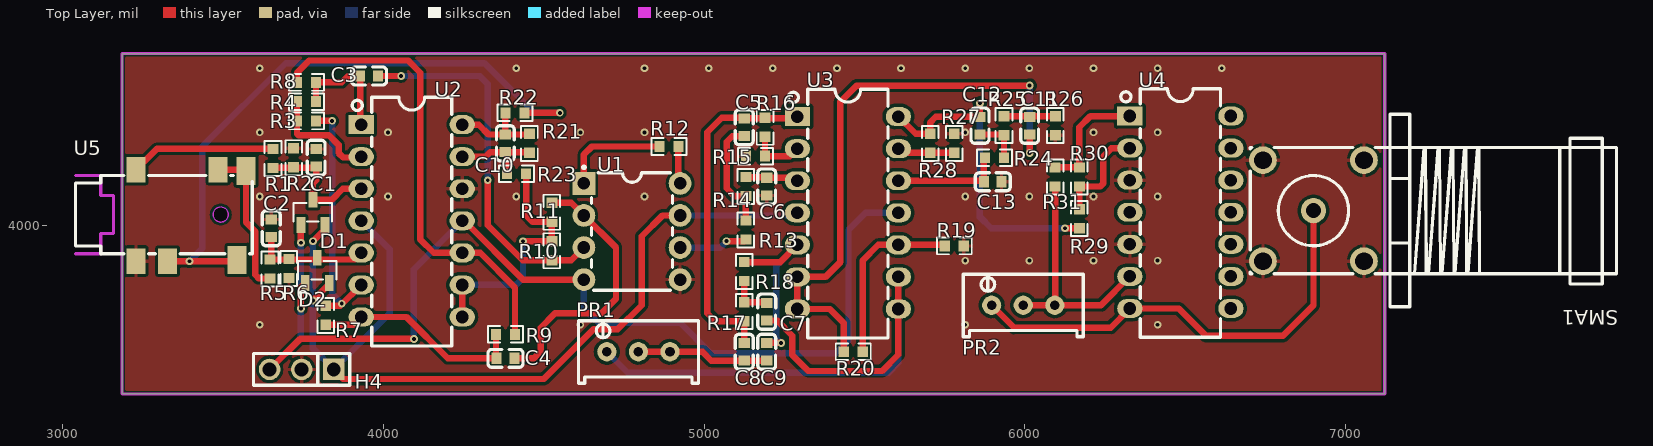
[diagram p0: Top Layer view]
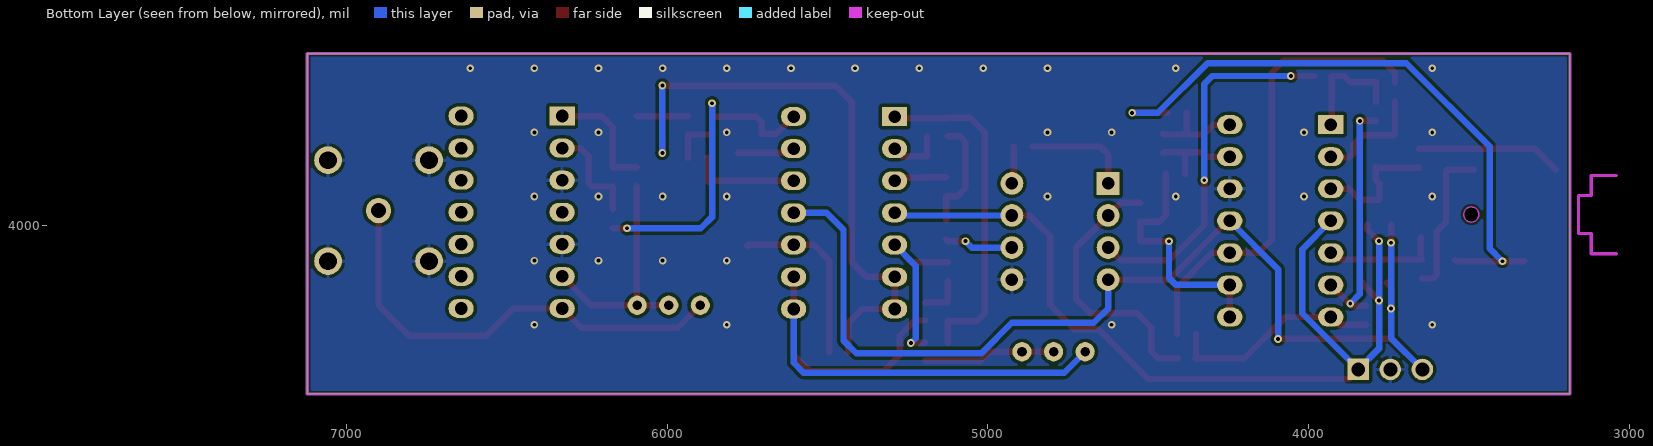
[diagram p1: Bottom Layer view, seen from below]
# Altium PCB MISC51578.pcbdoc
Units mil, origin at the board's own origin, x right, y up, seen from the top; angles counter-clockwise.
Board outline 3937.01 x 1061.35 mil, 2 copper layers (Top Layer, Bottom Layer), stack 62.206 mil thick; 55 components, 40 nets, 164 pads, 53 vias.

## Layer stack, top to bottom
Top Solder Mask Layer: solder mask 0.394, Dk 3.3
Top Layer: signal copper 1.379
Dielectric1: surface 59.449, FR4, Dk 4.5
Bottom Layer: signal copper 1.378
Bottom Solder Mask Layer: solder mask 0.394, Dk 3.3

## Board outline
3185,4535 3185,3473.65 7122.01,3473.65 7122.01,4535

## Design rules (kind name [scope] priority, off if disabled: settings)
BoardOutlineClearance copperThickness2oz_1 [All] p2 off: genericclearance=7.99 ignorepadtopadclearanceinfootprint=FALSE except(0: Arc-SplitContinuation Track-SplitContinuation SMDPad-SplitContinuation THPad-SplitContinuation Via-SplitContinuation Fill-SplitContinuation Region-SplitContinuation Poly-SplitContinuation Text-SplitContinuation Hole-SplitContinuation; 5.98: Arc-CutoutEdge SMDPad-CutoutEdge THPad-CutoutEdge Via-CutoutEdge Fill-CutoutEdge Region-CutoutEdge Text-CutoutEdge; 6.93: Hole-OutlineEdge Hole-CutoutEdge; 10: Poly-OutlineEdge Poly-CutoutEdge; 11.81: Arc-OutlineEdge Track-OutlineEdge SMDPad-OutlineEdge THPad-OutlineEdge Via-OutlineEdge Fill-OutlineEdge Region-OutlineEdge Text-OutlineEdge Track-CutoutEdge)
BoardOutlineClearance copperThickness1oz_1 [All] p4: genericclearance=4.02 ignorepadtopadclearanceinfootprint=FALSE except(0: Arc-SplitContinuation Track-SplitContinuation SMDPad-SplitContinuation THPad-SplitContinuation Via-SplitContinuation Fill-SplitContinuation Region-SplitContinuation Poly-SplitContinuation Text-SplitContinuation Hole-SplitContinuation; 6: SMDPad-CutoutEdge THPad-CutoutEdge Via-CutoutEdge Fill-CutoutEdge Region-CutoutEdge Text-CutoutEdge; 6.93: Hole-OutlineEdge Hole-CutoutEdge; 10: Poly-OutlineEdge Poly-CutoutEdge; 11.8: Arc-OutlineEdge Track-OutlineEdge SMDPad-OutlineEdge THPad-OutlineEdge Via-OutlineEdge Fill-OutlineEdge Region-OutlineEdge Text-OutlineEdge; 11.81: Arc-CutoutEdge Track-CutoutEdge)
Clearance copperThickness2oz [All] p1 off: gap=7.99 ignorepadtopadclearanceinfootprint=FALSE except(5.98: SMDPad-Track SMDPad-SMDPad THPad-Track SMDPad-THPad THPad-THPad Track-Via SMDPad-Via THPad-Via Via-Via Fill-Track Region-Track Fill-SMDPad Region-SMDPad Fill-THPad Region-THPad Fill-Via Region-Via Fill-Fill Fill-Region Region-Region Arc-Track Arc-SMDPad Arc-THPad Arc-Via Fill-Arc Region-Arc Arc-Arc Text-Track SMDPad-Text Text-THPad Text-Via Fill-Text Region-Text Arc-Text Text-Text; 6.93: Hole-Track Hole-SMDPad Hole-THPad Hole-Via Fill-Hole Region-Hole Hole-Arc Hole-Text; 10: Poly-Track Poly-SMDPad Poly-THPad Poly-Via Poly-Fill Poly-Region Poly-Poly Poly-Arc Poly-Text Poly-Hole)
Clearance copperThickness1oz [All] p3: gap=4.02 ignorepadtopadclearanceinfootprint=FALSE except(5.98: SMDPad-Track SMDPad-SMDPad THPad-Track SMDPad-THPad THPad-THPad Track-Via SMDPad-Via THPad-Via Via-Via Fill-Track Region-Track Fill-SMDPad Region-SMDPad Fill-THPad Region-THPad Fill-Via Region-Via Fill-Fill Fill-Region Region-Region; 6: Arc-Track Arc-SMDPad Arc-THPad Arc-Via Fill-Arc Region-Arc Arc-Arc Text-Track SMDPad-Text Text-THPad Text-Via Fill-Text Region-Text Arc-Text Text-Text; 6.93: Hole-Track Hole-SMDPad Hole-THPad Hole-Via Fill-Hole Region-Hole Hole-Arc Hole-Text; 10: Poly-Track Poly-SMDPad Poly-THPad Poly-Via Poly-Fill Poly-Region Poly-Poly Poly-Arc Poly-Text Poly-Hole)
DiffPairsRouting differentialPair [All] p1: maxlimit=6 minlimit=6 mostfreqgap=6 toplayer_minwidth=5 toplayer_prefwidth=10 toplayer_maxwidth=100 toplayer_mingap=6 toplayer_prefgap=6 toplayer_maxgap=6 bottomlayer_minwidth=5 bottomlayer_prefwidth=10 bottomlayer_maxwidth=100 bottomlayer_mingap=6 bottomlayer_prefgap=6 bottomlayer_maxgap=6 maxuncoupledlength=10
HoleToHoleClearance otherClearance [All] p1: gap=11.81 allowstackedmicrovias=TRUE
Length netLength [All] p1: minlimit=0 maxlimit=0
MatchedLengths netLengthTolerance [All] p1: tolerance=1000
PasteMaskExpansion pasteMaskExpansion [All] p1: expansion=0
PlaneConnect innerPlane [All] p1: planeconnectstyle=Relief reliefexpansion=20 reliefentries=4 reliefconductorwidth=10 reliefairgap=10
PolygonConnect copperRegion [(InNet('GND'))] p1: connectstyle=Relief reliefconductorwidth=10 reliefentries=4 polygonreliefangle="90 Angle" airgapwidth=10 via.connectstyle=Relief via.reliefconductorwidth=10 via.reliefentries=4 via.polygonreliefangle="90 Angle" via.airgapwidth=10
RoutingVias viaSize [All] p1: holewidth=12.01 width=24.02 viastyle="Through Hole" minholewidth=11.81 minwidth=19.68 maxholewidth=248.03 maxwidth=393.7
SolderMaskExpansion solderMaskExpansion [IsVia] p1: expansion=-1000 istentingtop=TRUE
SolderMaskExpansion solderMaskExpansion [All] p2: expansion=2 istentingtop=FALSE
Width copperThickness2oz_2 [All] p1 off: maxlimit=100 minlimit=8 preferedwidth=10
Width copperThickness1oz_2 [All] p2: maxlimit=100 minlimit=5 preferedwidth=10

## Components (designator, comment, footprint, x,y, rotation, side; value= is the part's Value field where it differs from the comment)
C1 "1nF" C0603 3790,4210 r270 top
C2 "1nF" C0603 3650,3990 r270 top
C3 "330nF" C0603 3955,4465 r0 top
C4 "330nF" C0603 4380.52,3584.47 r0 top
C5 "470nF" C0603 5125,4305 r90 top
C6 "470nF" C0603 5195,4120 r90 top
C7 "220nF" C0603 5195,3730 r90 top
C8 "100nF" C0603 5125,3605 r90 top
C9 "100nF" C0603 5195,3605 r270 top
C10 "22nF" C0603 4380,4255 r270 top
C11 "100nF" C0603 6015,4310 r270 top
C12 "470nF" C0603 5860,4310 r270 top
C13 "470nF" C0603 5900,4135 r180 top
D1 "BAV99" SOT-23-3_L2.9-W1.3-P1.90-LS2.4-BR 3780,4040 r270 top
D2 "BAV99" SOT-23-3_L2.9-W1.3-P1.90-LS2.4-BR 3793.75,3858.98 r270 top
H4 "" HDR-TH_3P-P2.54-V-M 3745,3550 r180 top
PR1 "10kΩ" R_3296 4795,3610 r0 top
PR2 "20kΩ" R_3296 5995,3755 r0 top
R1 "51K" R0603 3655.56,4208.01 r270 top
R2 "10M" R0603 3720,4210 r90 top
R3 "20K" R0603 3760,4325 r180 top
R4 "10K" R0603 3760,4385 r180 top
R5 "51K" R0603 3646.24,3863.01 r90 top
R6 "10M" R0603 3705,3865 r270 top
R7 "10K" R0603 3820.04,3718.69 r90 top
R8 "20K" R0603 3760,4445 r0 top
R9 "20K" R0603 4380.52,3659.47 r0 top
R10 "10MΩ" R0603 4525,3920 r270 top
R11 "10MΩ" R0603 4525,4040 r270 top
R12 "5K" R0603 4890,4245 r0 top
R13 "15K" R0603 5130,3985 r90 top
R14 "15K" R0603 5130,4120 r90 top
R15 "10K" R0603 5160,4215 r0 top
R16 "10K" R0603 5190,4305 r270 top
R17 "30K" R0603 5125,3730 r90 top
R18 "30K" R0603 5125,3855 r90 top
R19 "10K" R0603 5780,3935 r180 top
R20 "5K" R0603 5465,3605 r180 top
R21 "10M" R0603 4455,4255 r270 top
R22 "1M" R0603 4410,4350 r180 top
R23 "10K" R0603 4415,4160 r0 top
R24 "15K" R0603 5905,4210 r0 top
R25 "15K" R0603 5935,4310 r90 top
R26 "1M" R0603 6095,4310 r90 top
R27 "10K" R0603 5780,4255 r270 top
R28 "10K" R0603 5705,4255 r90 top
R29 "2K" R0603 6170,4020 r270 top
R30 "20K" R0603 6170,4150 r270 top
R31 "2K" R0603 6094.66,4150.34 r90 top
SMA1 "BNC-9.6" SMA-TH_5P_BNC-9.6 6900,4045 r180 top
U1 "AD620ANZ" DIP-8_L9.3-W6.4-P2.54-LS7.6-BL 4775,3980 r270 top
U2 "LM324NG" PDIP-14_L19.7-W6.6-P2.54-LS8.3-BL 4088.16,4013.35 r270 top
U3 "LM324NG" PDIP-14_L19.7-W6.6-P2.54-LS8.3-BL 5448.22,4038.35 r270 top
U4 "LM324NG" PDIP-14_L19.7-W6.6-P2.54-LS8.3-BL 6485,4040 r270 top
U5 "PJ-342 earphone jack" AUDIO-SMD_PJ-342_C9900012319 3400,4030 r0 top

## Footprints (in the part's own frame and the unit in brackets; to place one, negate y for a bottom-side part, rotate by r counter-clockwise, add the part's x,y. Pads: shape width x height; smd on the part's side, far side on the other; paste and mask are expansions set on the pad)
AUDIO-SMD_PJ-342_C9900012319 [mm]
  rect 1.5x2 smd paste+0 mask+0.05: 2(-4.35,-3.625) 3(-4.35,3.625) 6(2.15,3.625) 7(-1.85,-3.625)
  rect 1.5x2.2 smd paste+0 mask+0.05: 4(4.35,3.525) 5(3.65,-3.525)
  Board Outline Layer circle w0.003: c2.35,0.075 r0.6
  Board Outline Layer lines w0.254: -9.15,-3.025 -7.15,-3.025 -7.15,-1.425 -6.15,-1.425 -6.151,1.576 -7.149,1.576 -7.149,3.174 -9.15,3.174
  Board Outline Layer region: 2.95,0.075 2.891,-0.185 2.724,-0.394 2.484,-0.51 2.216,-0.51 1.976,-0.394 1.809,-0.185 1.75,0.075 1.75,0.075 1.809,0.335 1.976,0.544 2.216,0.66 2.484,0.66 2.724,0.544 2.891,0.335 2.95,0.075
  Board Outline Layer region: 2.95,0.075 2.941,-0.029 2.914,-0.13 2.87,-0.225 2.81,-0.311 2.736,-0.385 2.65,-0.445 2.555,-0.489 2.454,-0.516 2.35,-0.525 2.246,-0.516 2.145,-0.489 2.05,-0.445 1.964,-0.385 1.89,-0.311 1.83,-0.225 1.786,-0.13 1.759,-0.029 1.75,0.075 1.759,0.179 1.786,0.28 1.83,0.375 1.89,0.461 1.964,0.535 2.05,0.595 2.145,0.639 2.246,0.666 2.35,0.675 2.454,0.666 2.555,0.639 2.65,0.595 2.736,0.535 2.81,0.461 2.87,0.375 2.914,0.28 2.941,0.179
  Multi-Layer board cut-out: 2.95,0.075 2.891,-0.185 2.724,-0.394 2.484,-0.51 2.216,-0.51 1.976,-0.394 1.809,-0.185 1.75,0.075 1.75,0.075 1.809,0.335 1.976,0.544 2.216,0.66 2.484,0.66 2.724,0.544 2.891,0.335 2.95,0.075
  silkscreen extent -9.15,-3.03 4.85,3.17
C0603 [mm]
  rect 0.8x0.9 smd: 1(-0.7,0) 2(0.7,0)
  silkscreen extent -1.39,-0.71 1.39,0.71
DIP-8_L9.3-W6.4-P2.54-LS7.6-BL [mm]
  rect 1.8x1.8 hole 1: 1(-3.81,-3.81)
  round 1.8 hole 1: 2(-1.27,-3.81) 3(1.27,-3.81) 4(3.81,-3.81) 5(3.81,3.81) 6(1.27,3.81) 7(-1.27,3.81) 8(-3.81,3.81)
  silkscreen extent -5.18,-3.91 4.65,3.2
HDR-TH_3P-P2.54-V-M [mm]
  rect 1.7x1.7 hole 1.1: 1(-2.54,0)
  round 1.7 hole 1.1: 2(0,0) 3(2.54,0)
  silkscreen extent -3.81,-1.25 3.81,1.25
PDIP-14_L19.7-W6.6-P2.54-LS8.3-BL [mm]
  rect 1.5x2 hole 1: 1(-7.62,-4)
  oval 1.5x2 hole 1: 2(-5.08,-4) 3(-2.54,-4) 4(0,-4) 5(2.54,-4) 6(5.08,-4) 7(7.62,-4) 8(7.62,4) 9(5.08,4) 10(2.54,4) 11(0,4) 12(-2.54,4) 13(-5.08,4) 14(-7.62,4)
  silkscreen extent -9.78,-4.72 9.91,3.18
R0603 [mil]
  rect 31.75x34.02 smd paste-3937.01 mask+2: 1(-29.66,0) 2(29.66,0)
  silkscreen extent -55,-26 55,26
R_3296 [mil]
  round 60 hole 30 paste+0 mask+2: 1(-98.4,-5) 2(0,-5) 3(98.4,-5)
  silkscreen extent -187,-103 187,92
SMA-TH_5P_BNC-9.6 [mm]
  round 2.2 hole 1.4 paste+0 mask+0.05: 1(-4,4) 2(4,4) 3(4,-4) 4(-4,-4)
  round 2 hole 1.2 paste+0 mask+0.05: 5(0,0)
  silkscreen extent -24,-7.63 5,7.62
SOT-23-3_L2.9-W1.3-P1.90-LS2.4-BR [mm]
  rect 1.25x0.7 smd: 1(1,-0.95) 2(1,0.95) 3(-1,0)
  silkscreen extent -0.73,-1.53 0.73,1.53

## Via types
v1: diameter 24.02, hole 12, Top Layer to Bottom Layer, 53 vias

## Nets (pads, with @x,y where several pads share a name; then routed paths per layer and width w, separated by ;. In a path a pad name is that pad's centre, name@x,y a point inside that pad or via, vN(x,y) a via of type N, cw(c..) or ccw(c..) an arc to the next point about the centre after c; other vN are vias at no path point)
12V: D1.2 D2.2 H4.1 U1.7 U2.4 U3.4 | length 2940.5
  Top Layer w20: v1(3780,3765) 3831.15,3816.15 D2.2 ; v1(3780,3950) 3817.4,3987.4 D1.2 ; H4.1 3875,3520 4500,3520 4655,3675 4730,3675 4805,3750 4805,3965 4870,4030 U1.7
  Bottom Layer w20: v1(3780,3950) v1(3780,3765) 3780,3615 H4.1 4020,3725 4020,3924.04 U2.4 ; U1.7 5282.38,4030 U3.4
$1N2: C1.2 D1.3 R1.2 R2.1 U2.3 | length 408.1
  Top Layer w20: R1.2 3785.91,4178.35 C1.2 3790,4140 3780,4130 D1.3 3839.37,4079.37 3873.35,4113.35 U2.3
$1N14: R3.2 R4.2 U2.2 | length 346.9
  Top Layer w20: R4.2 R3.2 3730.34,4284.66 3735,4280 3830,4280 3860,4250 3860,4225 3874.14,4210.86 3928.19,4210.86 U2.2
$1N15: R3.1 R7.2 U2.6 | length 770.3
  Top Layer w20: R3.1 v1(3840,4325) ; R7.2 3865.68,3748.35 U2.6
  Bottom Layer w20: v1(3840,4325) 3840,3785 v1(3870,3755)
$1N21: C2.2 D2.3 R5.2 R6.1 U2.5 | length 364.3
  Top Layer w20: C2.2 3650,3896.43 R5.2 3910,3892.67 U2.5
$1N25: R8.1 R9.2 U2.10 | length 1469.2
  Top Layer w20: R8.1 3730.34,4475.34 3768.2,4513.2 4076.8,4513.2 4115,4475 4115,3955 4156.65,3913.35 U2.10 4301.65,3913.35 4410.19,3804.82 R9.2
$1N26: R10.1 R11.2 R23.2 U2.8 U2.9 | length 781.9
  Top Layer w20: U2.8 U2.9 ; v1(4435,3949.66) R10.1 R11.2 4464.66,4010.34 4444.66,4030.34 R23.2
  Bottom Layer w20: U2.9 4413.35,3813.35 4435,3835 v1(4435,3949.66)
$1N27: C3.2 R10.2 U1.3 | length 1154.6
  Top Layer w20: C3.2 v1(4055,4465) ; v1(4325,4140) 4325,4000 4434.66,3890.34 R10.2 4585.34,3890.34 U1.3
  Bottom Layer w20: v1(4055,4465) 4300,4465 4325,4440 v1(4325,4140)
$1N28: C3.1 R4.1 R8.2 U2.1 | length 359.1
  Top Layer w20: R4.1 R8.2 3870,4445 3890,4465 C3.1 3927.44,4316.6 U2.1
$1N30: C4.2 R11.1 U1.2 | length 855.5
  Top Layer w20: C4.2 4469.47,3584.47 4490,3605 4490,3680 4535,3725 4680,3725 4725,3770 4725,3930 U1.2 4585.34,4069.66 R11.1
$1N31: C4.1 R7.1 R9.1 U2.7 | length 672.3
  Top Layer w20: R7.1 3906.36,3689.03 U2.7 4071.65,3713.35 4200.53,3584.47 C4.1 4350.86,3586.57 R9.1
$1N35: R12.1 U1.1 | length 335.7
  Top Layer w20: U1.1 4625,4220 4650,4245 R12.1
$1N36: R12.2 U1.8 | length 117.2
  Top Layer w20: R12.2 4919.66,4135.34 U1.8
$1N37: R13.1 U1.6 | length 215.5
  Top Layer w20: v1(5070,3950) 5124.66,3950 R13.1
  Bottom Layer w20: U1.6 5050,3930 v1(5070,3950)
$1N40: C5.1 R13.2 R14.1 | length 353.1
  Top Layer w20: C5.1 5087.44,4277.44 5070,4260 5070,4115 5094.66,4090.34 R14.1 R13.2
$1N41: C6.2 R14.2 U3.3 | length 165.4
  Top Layer w20: R14.2 5192.9,4149.66 C6.2 5281.53,4147.56 U3.3
$1N44: R15.2 R16.2 U3.2 | length 171.2
  Top Layer w20: R16.2 5189.66,4275 R15.2 5267.38,4215 U3.2
$1N48: C5.2 C8.2 R16.1 R17.1 U3.1 | length 1060.8
  Top Layer w20: C8.2 R17.1 5034.66,3700.34 5010,3725 5010,4290 5055,4335 5122.56,4335 C5.2 5284.94,4332.56 U3.1
$1N49: C7.2 R17.2 R18.1 | length 136.5
  Top Layer w20: R18.1 R17.2 5192.9,3759.66 C7.2
$1N52: C8.1 C9.2 PR1.2 PR1.3 | length 411.4
  Top Layer w20: PR1.2 PR1.3 4995,3605 5022.56,3577.44 C8.1 C9.2
$1N53: C9.1 R18.2 U3.5 | length 572.2
  Top Layer w20: R18.2 5237.04,3884.66 U3.5 ; C9.1 v1(5240,3632.56)
  Bottom Layer w20: v1(5240,3632.56) 5225,3647.56 5225,3872.62 U3.5
$1N54: C7.1 PR1.1 U3.8 U3.9 | length 1891.1
  Top Layer w20: C7.1 5227.56,3702.44 5275,3655 5275,3595 5325,3545 5555,3545 5605.7,3595.7 U3.8 U3.9
  Bottom Layer w20: PR1.1 4761.6,3540 5575,3540 5605.7,3570.7 U3.8
$1N56: R19.2 R20.1 U3.10 | length 561.9
  Top Layer w20: R20.1 5494.66,3889.66 5543.35,3938.35 U3.10 5746.99,3938.35 R19.2
$1N61: C10.2 R21.2 R23.1 U2.13 | length 285.7
  Top Layer w20: U2.13 4318.35,4213.35 4332.44,4227.44 C10.2 ; R23.1 4385.34,4222.1 C10.2 ; R21.2 4452.9,4227.44 C10.2
$1N62: C10.1 R21.1 R22.2 U2.14 | length 290.6
  Top Layer w20: U2.14 4296.65,4313.35 4327.44,4282.56 C10.1 ; R22.2 4380.34,4282.9 C10.1 ; R21.1 4452.9,4282.56 C10.1
$1N63: R22.1 U5.5 U5.7 | length 1989.5
  Top Layer w20: U5.7 v1(3395.47,3887.28) 3539.76,3887.28 U5.5 ; R22.1 v1(4550,4350)
  Bottom Layer w20: v1(3395.47,3887.28) 3435.2,3927.01 3435.2,4245.2 3695,4505 4315,4505 4470,4350 v1(4550,4350)
$1N69: C13.2 R24.1 U3.12 | length 344.3
  Top Layer w20: U3.12 5869.09,4138.35 C13.2 5872.44,4207.1 R24.1
$1N73: C11.1 R25.2 R26.2 | length 160
  Top Layer w20: R25.2 R26.2
$1N74: C11.2 R20.2 U3.6 U3.7 | length 1884.1
  Top Layer w20: R20.2 5435.34,3694.66 5391.65,3738.35 U3.7 U3.6 5378.35,3838.35 5425,3885 5425,4385 5475,4435 v1(6015,4435) ; v1(6015,4225) C11.2
  Bottom Layer w20: v1(6015,4225) v1(6015,4435)
$1N76: C12.1 R28.2 R29.2 U3.14 | length 1041.2
  Top Layer w20: U3.14 5659.39,4284.66 R28.2 5705,4320 5722.56,4337.56 C12.1 v1(5860,4380) ; v1(6125,3990) 6169.66,3990 R29.2
  Bottom Layer w20: v1(5860,4380) 5860,4025 5895,3990 v1(6125,3990)
$1N77: C12.2 R24.2 R25.1 | length 146.4
  Top Layer w20: C12.2 5932.9,4282.44 R25.1 5935,4210.34 R24.2
$1N78: R27.2 R28.1 U3.13 | length 179.7
  Top Layer w20: U3.13 5618.71,4225.34 R28.1 R27.2
$1N79: R29.1 R30.2 U4.2 | length 327.6
  Top Layer w20: R29.1 R30.2 6235.34,4120.34 6245,4130 6245,4215 6270,4240 U4.2
$1N81: R30.1 R31.2 U4.1 | length 372.8
  Top Layer w20: R31.2 6169.66,4180 R30.1 6170,4305 6205,4340 U4.1
$1N83: PR2.2 PR2.3 R31.1 U4.6 | length 741
  Top Layer w20: PR2.2 PR2.3 ; R31.1 6094.66,3751.26 PR2.3 ; U4.6 6237.52,3750 PR2.3
$1N84: PR2.1 SMA1.5 U4.7 | length 1426.8
  Top Layer w20: PR2.1 5966.6,3680 6267.52,3680 U4.7 6480,3740 6565,3655 6805,3655 6900,3750 SMA1.5
$1N89: R1.1 U5.3 | length 453.7
  Top Layer w20: U5.3 3293.7,4237.67 R1.1
$1N90: R5.1 U5.4 U5.6 | length 475
  Top Layer w20: U5.6 3567.32,4172.72 U5.4 3571.26,4008.74 3600,3980 3600,3845 3611.65,3833.35 R5.1
-12V: D1.1 D2.1 H4.3 U1.4 U2.11 U3.11 | length 3464.1
  Top Layer w20: H4.3 3740,3645 v1(4095,3645) ; v1(3742.6,3740) 3742.6,3805.86 D2.1 ; v1(3742.6,3945) D1.1 ; U2.11 4251.65,4013.35 4435,3830 U1.4
  Bottom Layer w20: H4.3 3742.6,3647.6 v1(3742.6,3740) v1(3742.6,3945) ; v1(4095,3645) 4095,3862.71 U2.11 ; U1.4 4625,3740 4670,3695 4925,3695 5020,3600 5410,3600 5450,3640 5450,3985 5503.35,4038.35 U3.11
GND: C1.1 C2.1 C6.1 C13.1 H4.2 R2.2 R6.2 R15.1 R19.1 R26.1 R27.1 SMA1.1 SMA1.2 SMA1.3 SMA1.4 U1.5 U2.12 U4.3 U4.5 U5.2
  other v1: 3614.1,3689.1 4614.1,3689.1 5814.1,3689.1 6414.1,3689.1 5814.1,3889.1 6014.1,3889.1 6214.1,3889.1 6414.1,3889.1 3614.1,4089.1 4014.1,4089.1 4414.1,4089.1 4814.1,4089.1 5814.1,4089.1 6014.1,4089.1 6214.1,4089.1 6414.1,4089.1 3614.1,4289.1 4014.1,4289.1 4614.1,4289.1 4814.1,4289.1 5814.1,4289.1 6214.1,4289.1 6414.1,4289.1 3614.1,4489.1 4414.1,4489.1 4814.1,4489.1 5014.1,4489.1 5214.1,4489.1 5414.1,4489.1 5614.1,4489.1 5814.1,4489.1 6014.1,4489.1 6214.1,4489.1 6414.1,4489.1 6614.1,4489.1
pads on no net: U4.4 U4.8 U4.9 U4.10 U4.11 U4.12 U4.13 U4.14

## Polygon pours and split planes (outlines as drawn)
GND on Top Layer (solid, remove dead copper, pour order 0): 3020,4830 3020,3160 7435,3160 7435,4830
GND on Bottom Layer (solid, remove dead copper, pour order 2): 3000,4825 3000,3000 7750,3000 7750,4825

## Keep-outs
Board Outline Layer:
  the board outline again, w10

## Dimensions
7122.01,4585 to 3185,4585 on Document Layer